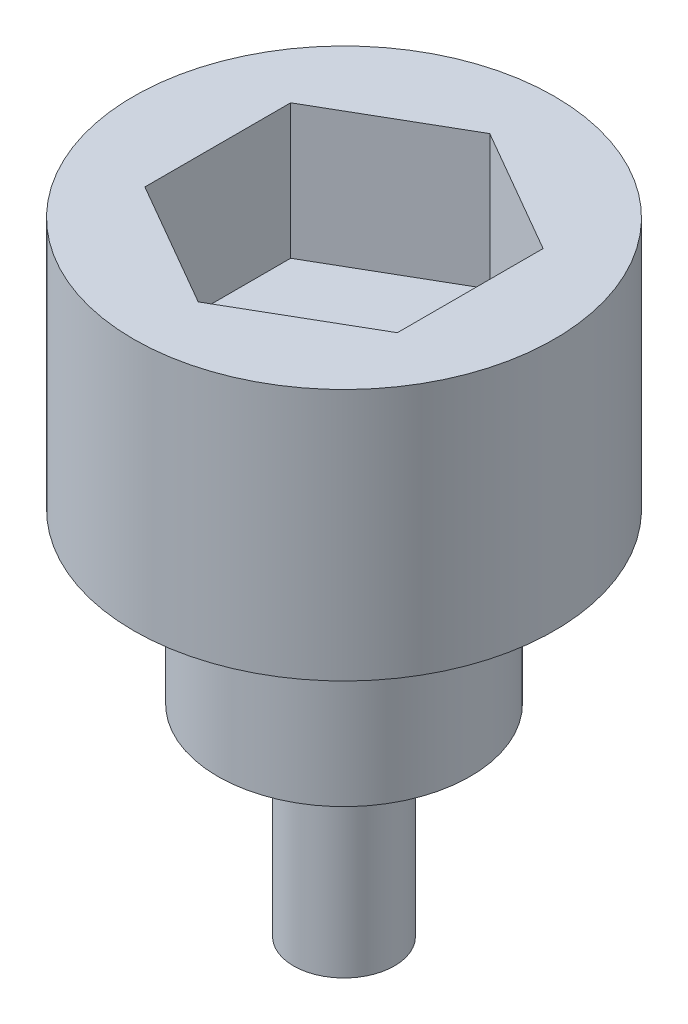
SolidWorks part; units mm, degrees
material "42CrMo"
ref_plane "Front Plane" through (0, 0, 0) normal (0, 0, 1) x (1, 0, 0)
ref_plane "Top Plane" through (0, 0, 0) normal (0, 1, 0) x (1, 0, 0)
ref_plane "Right Plane" through (0, 0, 0) normal (1, 0, 0) x (0, 0, -1)
sketch "Sketch1" plane through (0, 0, 0) normal (0, 1, 0) x (1, 0, 0)
  circle A0 centre (0, 0) radius 3
  dimension "D1" = 6
extrude "Boss-Extrude1" add sketch "Sketch1" along normal blind 12
cosmetic thread "Cosmetic Thread1" parameters "D2"=4.917
sketch "Sketch2" plane through (0, 12, 0) normal (0, 1, 0) x (1, 0, 0)
  circle A0 centre (0, 0) radius 7.5
  dimension "D1" = 15
extrude "Boss-Extrude2" add sketch "Sketch2" along normal blind 10
sketch "Sketch3" plane through (0, 22, 0) normal (0, 1, 0) x (1, 0, 0)
  circle A0 centre (0, 0) radius 12.5
  dimension "D1" = 25
extrude "Boss-Extrude3" add sketch "Sketch3" along normal blind 15
sketch "Sketch4" plane through (0, 37, 0) normal (0, 1, 0) x (1, 0, 0)
  line L1 (0, 8.6603) -> (-7.5, 4.3301)
  line L2 (-7.5, 4.3301) -> (-7.5, -4.3301)
  line L3 (-7.5, -4.3301) -> (0, -8.6603)
  line L4 (0, -8.6603) -> (7.5, -4.3301)
  line L5 (7.5, -4.3301) -> (7.5, 4.3301)
  line L6 (7.5, 4.3301) -> (0, 8.6603)
  circle A0 centre (0, 0) radius 7.5 construction
  dimension "D2" = 15
extrude "Cut-Extrude1" cut sketch "Sketch4" against normal blind 8
